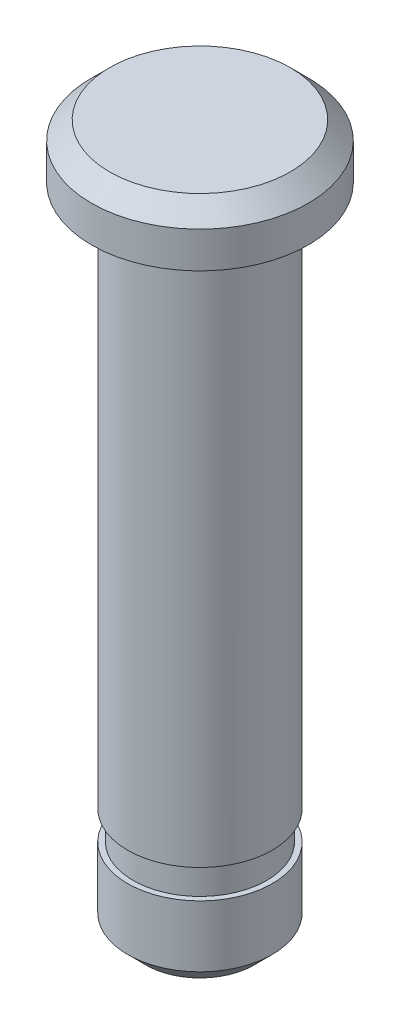
from build123d import *

# Parameters (mm, degrees)
SKETCH1_R           = 3
BOSS_EXTRUDE1_DEPTH = 1.5
SKETCH2_R           = 2
BOSS_EXTRUDE2_DEPTH = 18
SKETCH3_W           = 0.15
SKETCH3_H           = 0.8
CHAMFER1_SIZE       = 0.5


with BuildPart() as part:
    # Sketch1 → Boss-Extrude1 (new body)
    with BuildSketch(Plane(origin=(0, 0, 0), x_dir=(1, 0, 0), z_dir=(0, 1, 0))):
        with Locations(Location((0, 0, 0), (0, 0, 270))):
            Circle(SKETCH1_R)
    extrude(amount=BOSS_EXTRUDE1_DEPTH)

    # Sketch2 → Boss-Extrude2 (add)
    with BuildSketch(Plane.XZ):
        with Locations(Location((0, 0, 0), (0, 0, 90))):
            Circle(SKETCH2_R)
    extrude(amount=BOSS_EXTRUDE2_DEPTH)

    # Sketch3 → Cut-Revolve1 (revolve, cut)
    with BuildSketch(Plane(origin=(0, 0, 0), x_dir=(0, 0, -1), z_dir=(1, 0, 0))):
        with Locations((1.925, -15.4)):
            Rectangle(SKETCH3_W, SKETCH3_H)
    revolve(axis=Axis((0, -16.563495901, 0), (0, 1, 0)), mode=Mode.SUBTRACT)

    # Chamfer1
    chamfer1_edges = [part.edges().sort_by_distance(p)[0] for p in [
        (0, 1.5, -3),
        (0, -18, -2),
    ]]
    chamfer(chamfer1_edges, length=CHAMFER1_SIZE)


solid = part.part
